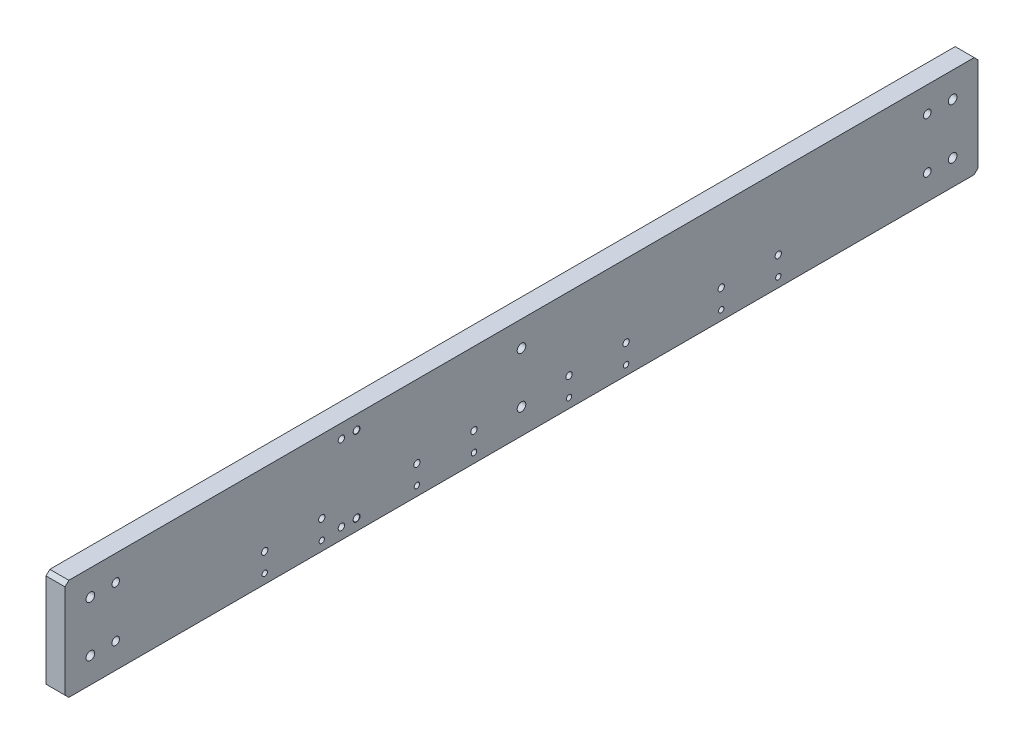
from build123d import *

# Parameters (mm, degrees)
SKETCH1_W                        = 720
SKETCH1_H                        = 80
BOSS_EXTRUDE1_DEPTH              = 15
M5_TAPPED_HOLE1_D                = 4.2
M5_TAPPED_HOLE1_DEPTH            = 12.4
M5_TAPPED_HOLE1_TIP              = 1.2618073
F_5_0MM_BLIND_HOLE_1_D           = 5
F_5_0MM_BLIND_HOLE_1_DEPTH       = 6
F_5_0MM_BLIND_HOLE_1_TIP         = 1.502151548
M8_TAPPED_HOLE1_D                = 6.8
M8_TAPPED_HOLE1_DEPTH            = 19.75
M8_TAPPED_HOLE1_TIP              = 2.042926105
F_6_0MM_BLIND_HOLE_1_D           = 6
F_6_0MM_BLIND_HOLE_1_DEPTH       = 8
F_6_0MM_BLIND_HOLE_1_TIP         = 1.802581857
M8_TAPPED_HOLE2_D                = 6.8
M8_TAPPED_HOLE2_DEPTH            = 19.75
M8_TAPPED_HOLE2_TIP              = 2.042926105
M6_TAPPED_HOLE1_D                = 5
M6_TAPPED_HOLE1_DEPTH            = 15
M6_TAPPED_HOLE1_TIP              = 1.502151548
F_5_0MM_BLIND_HOLE_2_D           = 5
F_5_0MM_BLIND_HOLE_2_DEPTH       = 8
F_5_0MM_BLIND_HOLE_2_CSINK_D     = 5.4
F_5_0MM_BLIND_HOLE_2_CSINK_ANGLE = 90
F_5_0MM_BLIND_HOLE_2_TIP         = 1.502151548
CHAMFER1_SIZE                    = 3


with BuildPart() as part:
    # Sketch1 → Boss-Extrude1 (new body)
    with BuildSketch(Plane(origin=(0, 0, 0), x_dir=(0, 0, -1), z_dir=(1, 0, 0))):
        Rectangle(SKETCH1_W, SKETCH1_H)
    extrude(amount=BOSS_EXTRUDE1_DEPTH)

    # M5 Tapped Hole1
    with Locations(Plane(origin=(15, 0, 0), x_dir=(0, 0, -1), z_dir=(1, 0, 0))):
        with Locations((202.5, -32.5), (157.5, -32.5), (82.5, -32.5), (37.5, -32.5), (-37.5, -32.5), (-82.5, -32.5), (-157.5, -32.5), (-202.5, -32.5)):
            Hole(M5_TAPPED_HOLE1_D / 2, depth=M5_TAPPED_HOLE1_DEPTH)
            with Locations((0, 0, -(M5_TAPPED_HOLE1_DEPTH + M5_TAPPED_HOLE1_TIP / 2))):  # 118° drill point
                Cone(0, M5_TAPPED_HOLE1_D / 2, M5_TAPPED_HOLE1_TIP, mode=Mode.SUBTRACT)

    # Ø5.0mm blind hole 1
    with Locations(Plane(origin=(15, 0, 0), x_dir=(0, 0, -1), z_dir=(1, 0, 0))):
        with Locations((-202.5, -17.5), (-157.5, -17.5), (-82.5, -17.5), (-37.5, -17.5), (37.5, -17.5), (82.5, -17.5), (157.5, -17.5), (202.5, -17.5)):
            Hole(F_5_0MM_BLIND_HOLE_1_D / 2, depth=F_5_0MM_BLIND_HOLE_1_DEPTH)
            with Locations((0, 0, -(F_5_0MM_BLIND_HOLE_1_DEPTH + F_5_0MM_BLIND_HOLE_1_TIP / 2))):  # 118° drill point
                Cone(0, F_5_0MM_BLIND_HOLE_1_D / 2, F_5_0MM_BLIND_HOLE_1_TIP, mode=Mode.SUBTRACT)

    # M8 Tapped Hole1
    with Locations(Plane(origin=(15, 0, 0), x_dir=(0, 0, -1), z_dir=(1, 0, 0))):
        with Locations((340, 20), (-340, 20), (-340, -20), (340, -20)):
            Hole(M8_TAPPED_HOLE1_D / 2, depth=M8_TAPPED_HOLE1_DEPTH)
            with Locations((0, 0, -(M8_TAPPED_HOLE1_DEPTH + M8_TAPPED_HOLE1_TIP / 2))):  # 118° drill point
                Cone(0, M8_TAPPED_HOLE1_D / 2, M8_TAPPED_HOLE1_TIP, mode=Mode.SUBTRACT)

    # Ø6.0mm blind hole 1
    with Locations(Plane(origin=(15, 0, 0), x_dir=(0, 0, -1), z_dir=(1, 0, 0))):
        with Locations((320, -20), (-320, 20), (-320, -20), (320, 20)):
            Hole(F_6_0MM_BLIND_HOLE_1_D / 2, depth=F_6_0MM_BLIND_HOLE_1_DEPTH)
            with Locations((0, 0, -(F_6_0MM_BLIND_HOLE_1_DEPTH + F_6_0MM_BLIND_HOLE_1_TIP / 2))):  # 118° drill point
                Cone(0, F_6_0MM_BLIND_HOLE_1_D / 2, F_6_0MM_BLIND_HOLE_1_TIP, mode=Mode.SUBTRACT)

    # M8 Tapped Hole2
    with Locations(Plane(origin=(15, 0, 0), x_dir=(0, 0, -1), z_dir=(1, 0, 0))):
        with Locations((0, -20), (0, 20)):
            Hole(M8_TAPPED_HOLE2_D / 2, depth=M8_TAPPED_HOLE2_DEPTH)
            with Locations((0, 0, -(M8_TAPPED_HOLE2_DEPTH + M8_TAPPED_HOLE2_TIP / 2))):  # 118° drill point
                Cone(0, M8_TAPPED_HOLE2_D / 2, M8_TAPPED_HOLE2_TIP, mode=Mode.SUBTRACT)

    # M6 Tapped Hole1
    with Locations(Plane(origin=(15, 0, 0), x_dir=(0, 0, -1), z_dir=(1, 0, 0))):
        with Locations((-142.05, 29), (-142.05, -31)):
            Hole(M6_TAPPED_HOLE1_D / 2, depth=M6_TAPPED_HOLE1_DEPTH)
            with Locations((0, 0, -(M6_TAPPED_HOLE1_DEPTH + M6_TAPPED_HOLE1_TIP / 2))):  # 118° drill point
                Cone(0, M6_TAPPED_HOLE1_D / 2, M6_TAPPED_HOLE1_TIP, mode=Mode.SUBTRACT)

    # Ø5.0mm blind hole 2
    with Locations(Plane(origin=(15, 0, 0), x_dir=(0, 0, -1), z_dir=(1, 0, 0))):
        with Locations((-130.05, -31), (-130.05, 29)):
            CounterSinkHole(F_5_0MM_BLIND_HOLE_2_D / 2, F_5_0MM_BLIND_HOLE_2_CSINK_D / 2, depth=F_5_0MM_BLIND_HOLE_2_DEPTH, counter_sink_angle=F_5_0MM_BLIND_HOLE_2_CSINK_ANGLE)
            with Locations((0, 0, -(F_5_0MM_BLIND_HOLE_2_DEPTH + F_5_0MM_BLIND_HOLE_2_TIP / 2))):  # 118° drill point
                Cone(0, F_5_0MM_BLIND_HOLE_2_D / 2, F_5_0MM_BLIND_HOLE_2_TIP, mode=Mode.SUBTRACT)

    # Chamfer1
    chamfer1_edges = [part.edges().sort_by_distance(p)[0] for p in [
        (7.5, -40, -360),
        (7.5, -40, 360),
        (7.5, 40, 360),
        (7.5, 40, -360),
    ]]
    chamfer(chamfer1_edges, length=CHAMFER1_SIZE)


solid = part.part
